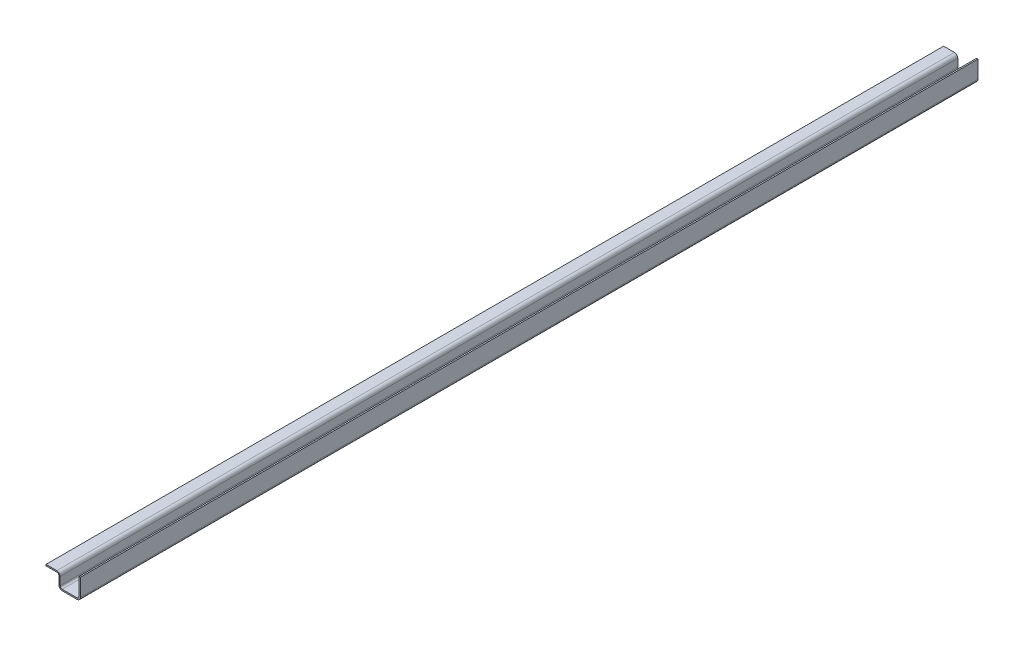
SolidWorks part; units mm, degrees
ref_plane "前视基准面" through (0, 0, 0) normal (0, 0, 1) x (1, 0, 0)
ref_plane "上视基准面" through (0, 0, 0) normal (0, 1, 0) x (1, 0, 0)
ref_plane "右视基准面" through (0, 0, 0) normal (1, 0, 0) x (0, 0, -1)
sketch "草图1" plane through (0, 0, 0) normal (0, 0, 1) x (1, 0, 0)
  line L0 (0, 0) -> (-30, 0)
  line L1 (-30, 0) -> (-30, 20)
  line L2 (-30, 20) -> (-50, 20)
  line L3 (0, 0) -> (0, 30)
  dimension "D1" = 30
  dimension "D2" = 30
  dimension "D3" = 20
  dimension "D4" = 20
extrude "拉伸-薄壁1" add sketch "草图1" along normal mid plane 1331 thin thin type mid plane wall 2
